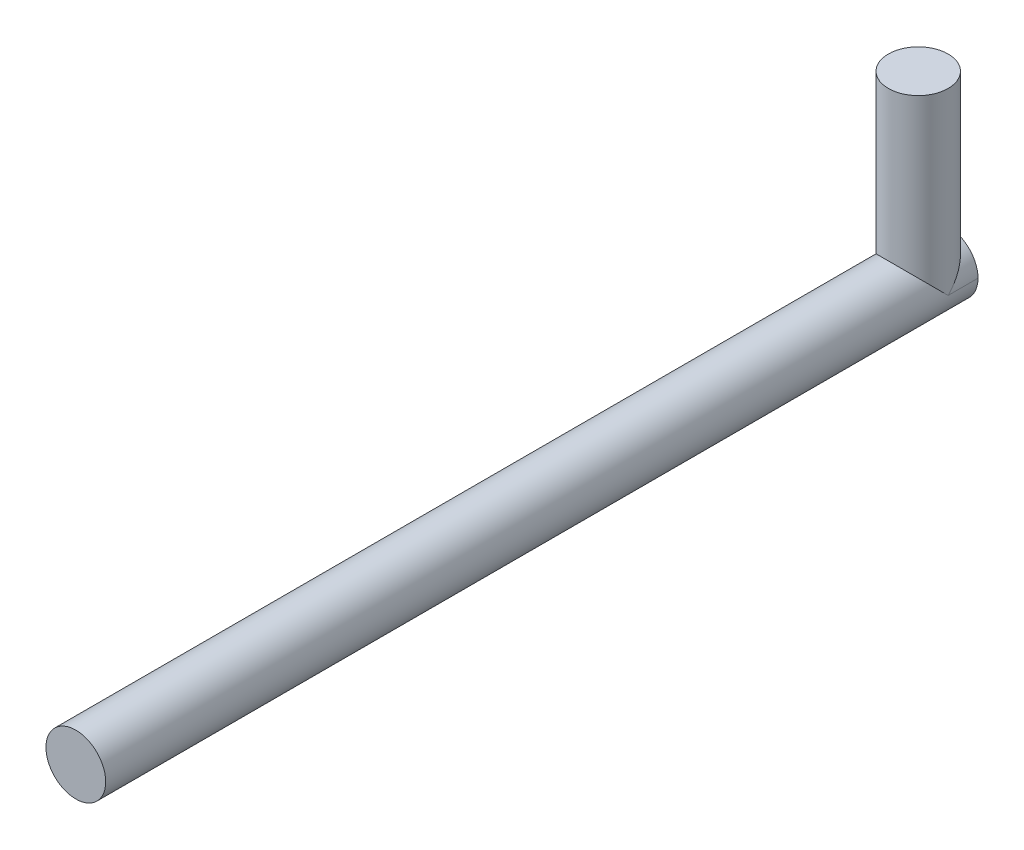
SolidWorks part; units mm, degrees
ref_plane "前视基准面" through (0, 0, 0) normal (0, 0, 1) x (1, 0, 0)
ref_plane "上视基准面" through (0, 0, 0) normal (0, 1, 0) x (1, 0, 0)
ref_plane "右视基准面" through (0, 0, 0) normal (1, 0, 0) x (0, 0, -1)
sketch "草图1" plane through (0, 0, 0) normal (0, 0, 1) x (1, 0, 0)
  circle A0 centre (0, 0) radius 2.5
  dimension "D1" = 5
extrude "凸台-拉伸1" add sketch "草图1" along normal blind 73 contours A0
sketch "草图2" plane through (0, 0, 0) normal (0, 1, 0) x (1, 0, 0)
  circle A0 centre (0, -2.5) radius 2.5
  dimension "D1" = 5
extrude "凸台-拉伸2" add sketch "草图2" along normal blind 15
